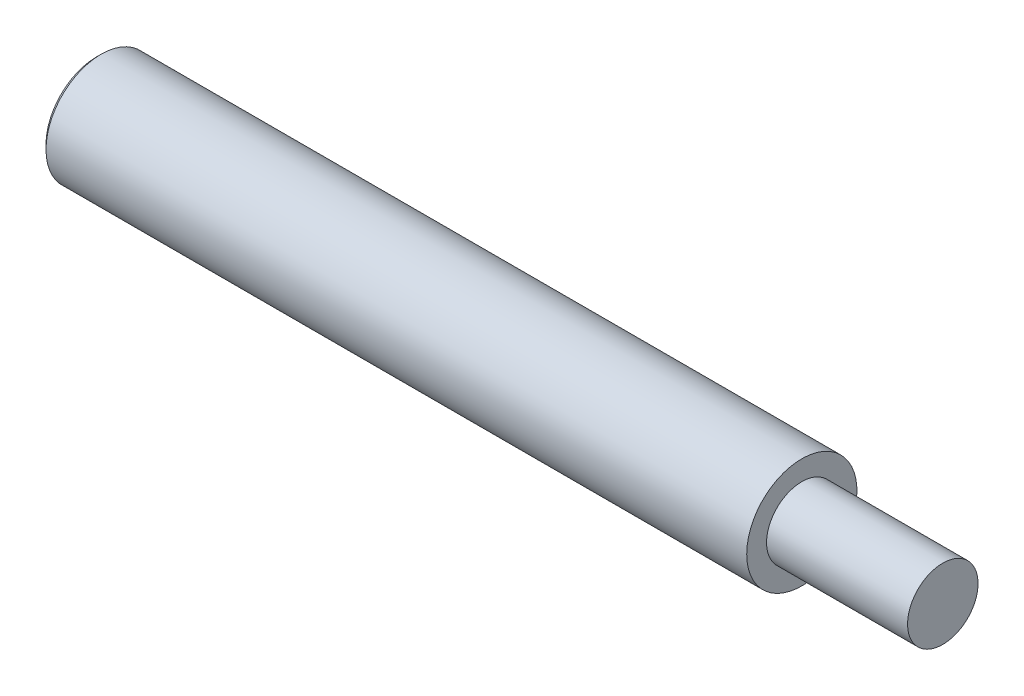
SolidWorks part; units mm, degrees
material "Q235A"
ref_plane "Front Plane" through (0, 0, 0) normal (0, 0, 1) x (1, 0, 0)
ref_plane "Top Plane" through (0, 0, 0) normal (0, 1, 0) x (1, 0, 0)
ref_plane "Right Plane" through (0, 0, 0) normal (1, 0, 0) x (0, 0, -1)
sketch "Sketch1" plane through (0, 0, 0) normal (0, 0, 1) x (1, 0, 0)
  line L0 (0, 0) -> (234.1079, 0) construction
  line L1 (0, 0) -> (0, 12.5)
  line L2 (0, 12.5) -> (160, 12.5)
  line L3 (160, 12.5) -> (160, 8)
  line L4 (160, 8) -> (192, 8)
  line L5 (192, 8) -> (192, 0)
  line L6 (0, 0) -> (192, 0)
  dimension "D1" = 25
  dimension "D2" = 16
  dimension "D3" = 32
  dimension "D4" = 160
revolve "Revolve1" add sketch "Sketch1" angle 360 about L0
chamfer "Chamfer1" distance 1 angle 45 1 edges at (0, 0, 12.5)
